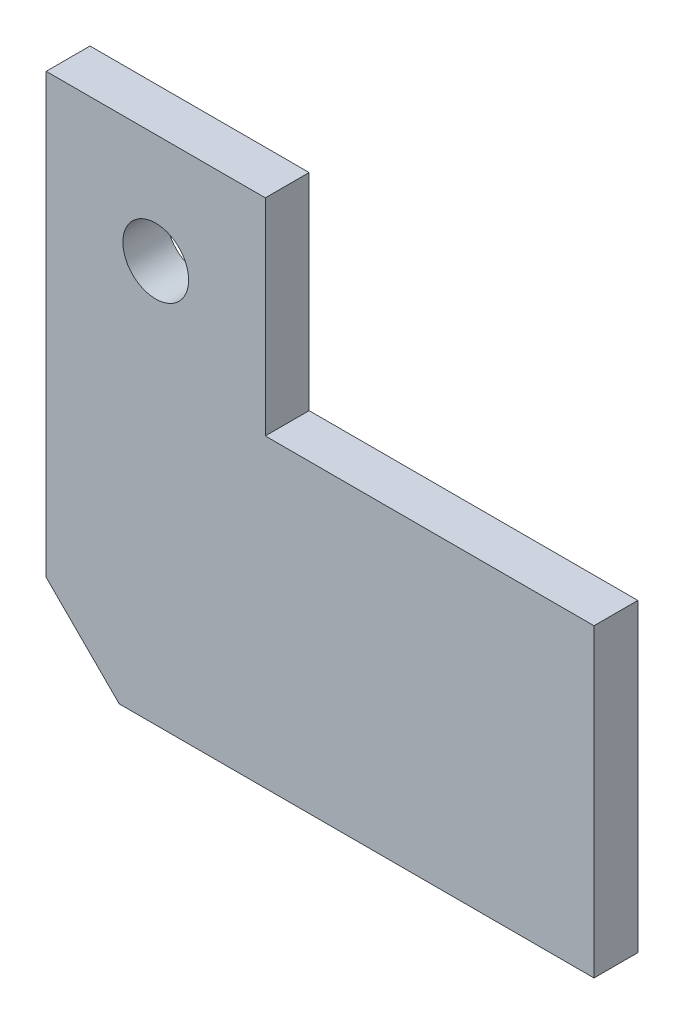
SolidWorks part; units mm, degrees
material "Q235B"
ref_plane "Front" through (0, 0, 0) normal (0, 0, 1) x (1, 0, 0)
ref_plane "Top" through (0, 0, 0) normal (0, 1, 0) x (1, 0, 0)
ref_plane "Right" through (0, 0, 0) normal (1, 0, 0) x (0, 0, -1)
sketch "Sketch1" plane through (0, 0, 0) normal (0, 0, 1) x (1, 0, 0)
  line L0 (-33.5216, -18.6225) -> (-33.5216, 51.3775)
  line L1 (-33.5216, 51.3775) -> (-3.5216, 51.3775)
  line L2 (-3.5216, 51.3775) -> (-3.5216, 23.1445)
  line L3 (-3.5216, 23.1445) -> (41.4784, 23.1445)
  line L4 (41.4784, 23.1445) -> (41.4784, -18.6225)
  line L5 (41.4784, -18.6225) -> (-33.5216, -18.6225)
  dimension "D1" = 75
  dimension "D2" = 70
  dimension "D3" = 30
extrude "Boss-Extrude1" add sketch "Sketch1" along normal blind 6
sketch "Sketch2" plane through (0, 0, 6) normal (0, 0, 1) x (1, 0, 0)
  line L0 (-3.5216, 51.3775) -> (-33.5216, 51.3775) construction
  line L1 (-18.5216, 51.3775) -> (-18.5216, 26.5641) construction
  circle A0 centre (-18.5216, 36.3775) radius 4.5
  dimension "D1" = 15
  dimension "D2" = 9
extrude "Cut-Extrude1" cut sketch "Sketch2" against normal up to next
chamfer "Chamfer1" distance 10 angle 45 1 edges at (-33.5216, -18.6225, 3)
equation "\"零件重量\"= IIF ( \"SW-质量\" > 100 , int ( \"SW-质量\" ) , \"SW-质量\" )"
